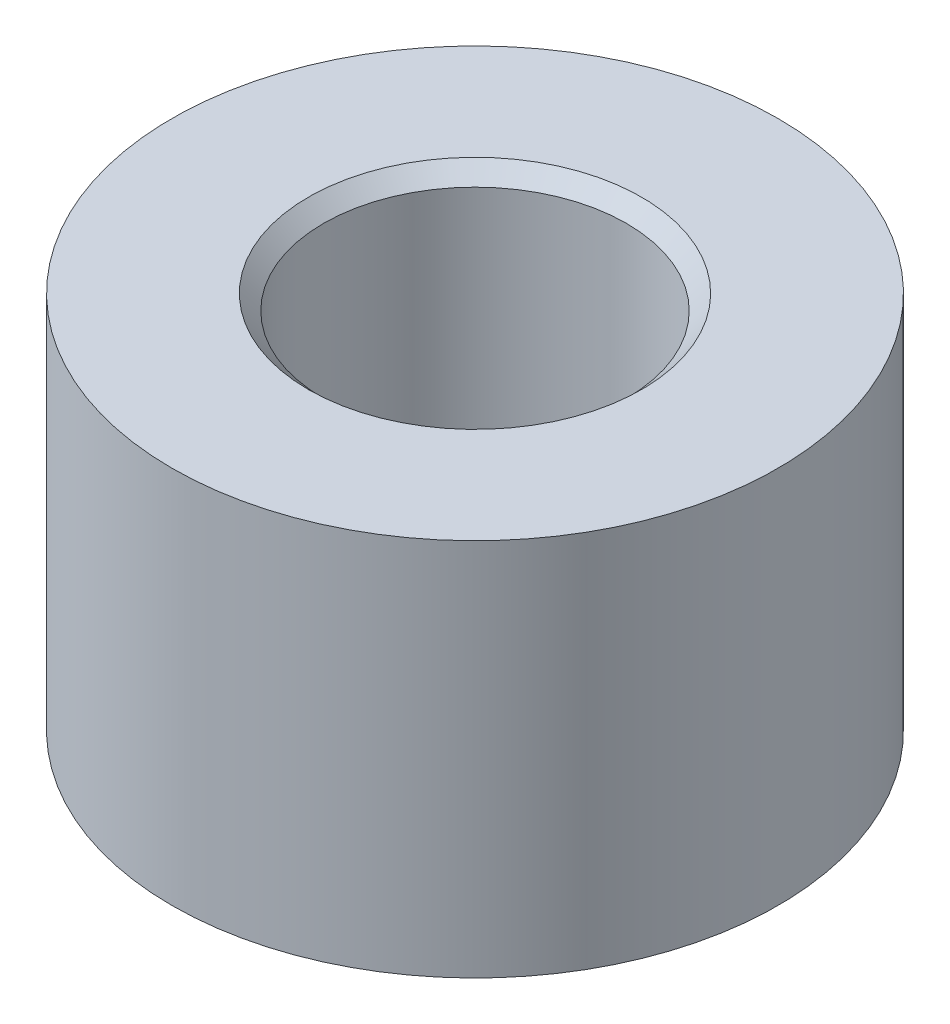
SolidWorks part; units mm, degrees
material "AISI 304"
ref_plane "前视基准面" through (0, 0, 0) normal (0, 0, 1) x (1, 0, 0)
ref_plane "上视基准面" through (0, 0, 0) normal (0, 1, 0) x (1, 0, 0)
ref_plane "右视基准面" through (0, 0, 0) normal (1, 0, 0) x (0, 0, -1)
sketch "草图1" plane through (0, 0, 0) normal (0, 1, 0) x (1, 0, 0)
  circle A0 centre (0, 0) radius 2
  circle A1 centre (0, 0) radius 1
  dimension "D1" = 4
  dimension "D2" = 2
extrude "凸台-拉伸1" add sketch "草图1" along normal blind 2.5
chamfer "C0.1 倒角1" distance 0.1 angle 45 2 edges at (0, 0, 1) (0, 2.5, 1)
